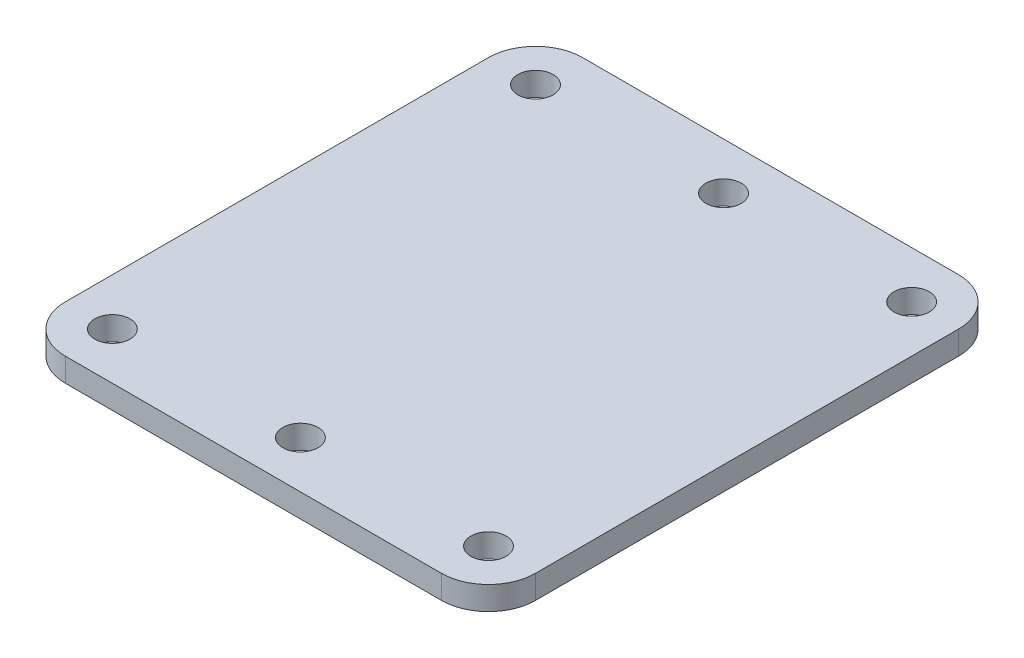
from build123d import *

# Parameters (mm, degrees)
SKETCH1_W            = 200
SKETCH1_H            = 220
BOSS_EXTRUDE1_DEPTH  = 5
SKETCH2_R            = 7.5
CUT_EXTRUDE1_DEPTH   = 10
LPATTERN1_COUNT      = 2
LPATTERN1_PITCH      = 180
LPATTERN1_COUNT_DIR2 = 3
LPATTERN1_PITCH_DIR2 = 80
FILLET1_R            = 20


with BuildPart() as part:
    # Sketch1 → Boss-Extrude1 (new, symmetric)
    with BuildSketch(Plane(origin=(0, 0, 0), x_dir=(1, 0, 0), z_dir=(0, 1, 0))):
        Rectangle(SKETCH1_W, SKETCH1_H)
    extrude(amount=BOSS_EXTRUDE1_DEPTH, both=True)

    # Sketch2 → Cut-Extrude1 (cut)
    with BuildSketch(Plane(origin=(0, 5, 0), x_dir=(1, 0, 0), z_dir=(0, 1, 0))):
        with Locations(Location((80, 90, 0), (0, 0, 270))):
            Circle(SKETCH2_R)
    cut_extrude1 = extrude(amount=-CUT_EXTRUDE1_DEPTH, mode=Mode.SUBTRACT)

    # LPattern1: Cut-Extrude1 2 × 3
    with Locations(*[(-j * LPATTERN1_PITCH_DIR2, 0, i * LPATTERN1_PITCH) for i in range(LPATTERN1_COUNT) for j in range(LPATTERN1_COUNT_DIR2) if (i, j) != (0, 0)]):
        add(cut_extrude1, mode=Mode.SUBTRACT)

    # Fillet1
    fillet1_edges = [part.edges().sort_by_distance(p)[0] for p in [
        (100, 0, 110),
        (-100, 0, 110),
        (-100, 0, -110),
        (100, 0, -110),
    ]]
    fillet(fillet1_edges, radius=FILLET1_R)


solid = part.part
